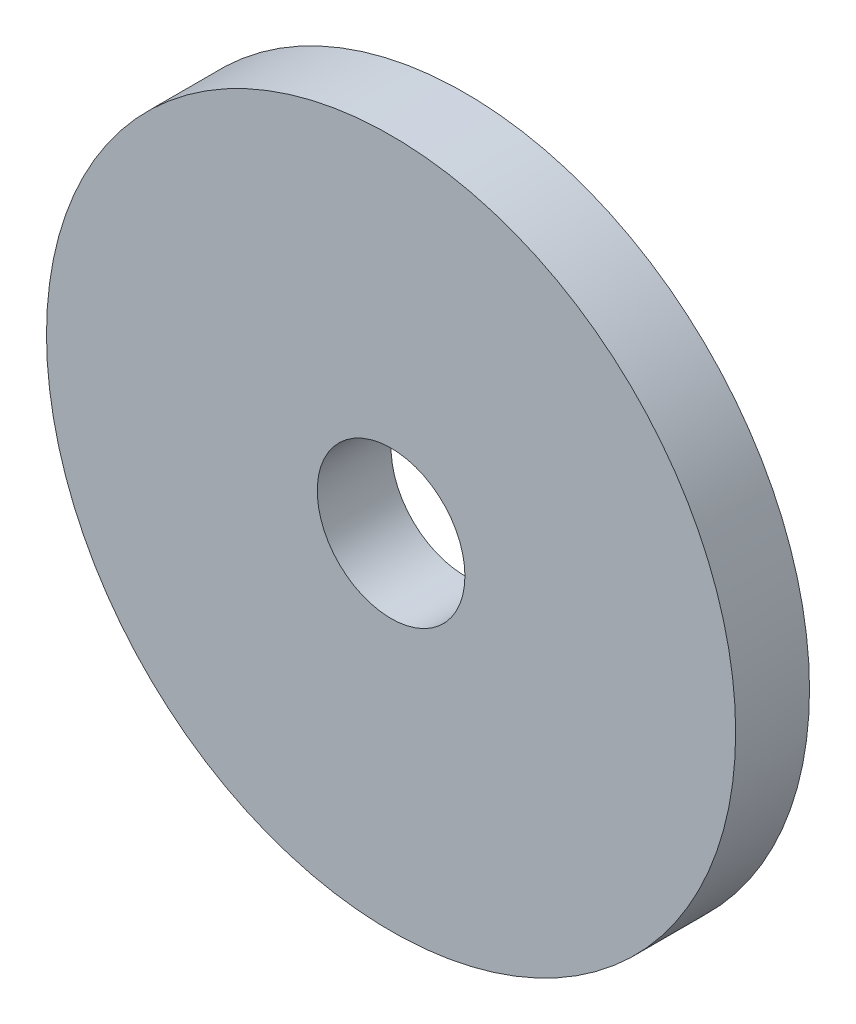
from build123d import *

# Parameters (mm, degrees)
SKETCH1_R           = 14
SKETCH1_R_2         = 3
BOSS_EXTRUDE1_DEPTH = 3


with BuildPart() as part:
    # Sketch1 → Boss-Extrude1 (new body)
    with BuildSketch(Plane.XY):
        Circle(SKETCH1_R)
        Circle(SKETCH1_R_2, mode=Mode.SUBTRACT)
    extrude(amount=BOSS_EXTRUDE1_DEPTH)


solid = part.part
